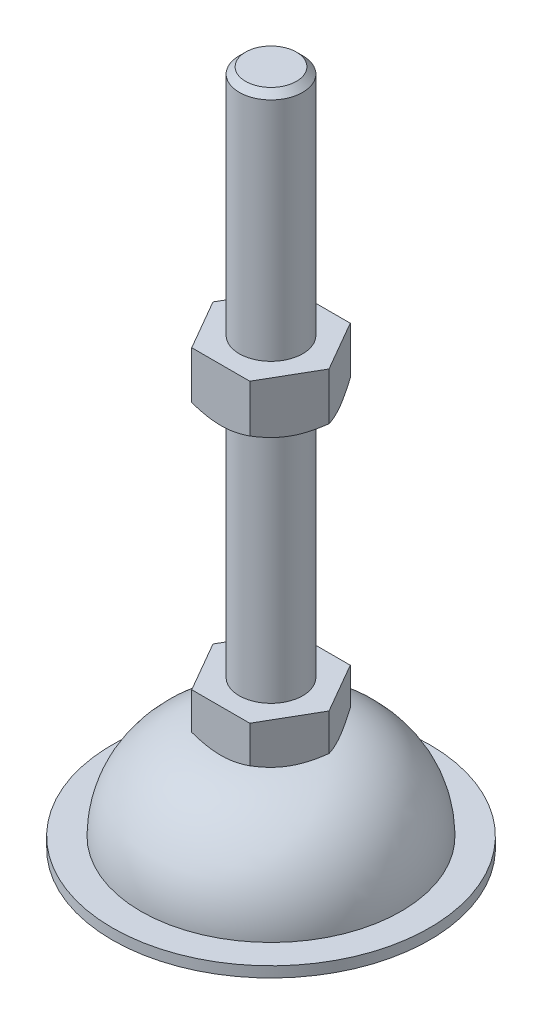
SolidWorks part; units mm, degrees
ref_plane "Front Plane" through (0, 0, 0) normal (0, 0, 1) x (1, 0, 0)
ref_plane "Top Plane" through (0, 0, 0) normal (0, 1, 0) x (1, 0, 0)
ref_plane "Right Plane" through (0, 0, 0) normal (1, 0, 0) x (0, 0, -1)
sketch "Sketch1" plane through (0, 0, 0) normal (1, 0, 0) x (0, 0, -1)
  line L0 (0, 0) -> (0, 128) construction
  line L1 (0, 128) -> (6, 128)
  line L2 (6, 128) -> (6, 20)
  line L3 (0, 0) -> (30, 0)
  line L4 (30, 0) -> (30, 2)
  line L5 (30, 2) -> (24.6, 2)
  line L6 (6, 20) -> (6.6, 20)
  line L8 (0, 84) -> (9.5, 84)
  line L9 (0, 84) -> (0, 74)
  line L10 (0, 74) -> (9.5, 74)
  line L11 (9.5, 84) -> (9.5, 74)
  line L12 (0, 28) -> (9.5, 28)
  line L13 (0, 28) -> (0, 20)
  line L14 (0, 20) -> (9.5, 20)
  line L15 (9.5, 28) -> (9.5, 20)
  arc A1 (24.6, 2) -> (6.6, 20) centre (6.6, 2) ccw
  point P18 (6, 74)
  dimension "D1" = 0.6
  dimension "M" = 12
  dimension "D" = 60
  dimension "e1" = 8
  dimension "e2" = 10
  dimension "E" = 18
  dimension "t" = 2
  dimension "B" = 19
  dimension "A" = 100
sketch "Sketch2" plane through (0, 0, 0) normal (1, 0, 0) x (0, 0, -1)
  line L0 (0, 128) -> (6, 128) construction
  line L1 (6, 128) -> (6, 20) construction
  line L2 (6, 20) -> (6.6, 20) construction
  line L3 (30, 2) -> (24.6, 2) construction
  line L4 (30, 0) -> (30, 2) construction
  line L5 (0, 0) -> (30, 0) construction
  line L6 (0, 128) -> (6, 128)
  line L7 (6, 128) -> (6, 20)
  line L8 (6, 20) -> (6.6, 20)
  line L9 (30, 2) -> (24.6, 2)
  line L10 (30, 0) -> (30, 2)
  line L11 (0, 0) -> (30, 0)
  line L12 (0, 128) -> (0, 0)
  arc A0 (24.6, 2) -> (6.6, 20) centre (6.6, 2) ccw construction
  arc A1 (24.6, 2) -> (6.6, 20) centre (6.6, 2) ccw
revolve "Revolve1" add sketch "Sketch2" angle 360 mid plane about L12
cosmetic thread "Cosmetic Thread1" parameters "D2"=11.9
chamfer "Chamfer1" distance 1.2 angle 45 1 edges at (0, 128, 6)
sketch "Sketch3" plane through (0, 0, 0) normal (0, 1, 0) x (1, 0, 0)
  line L1 (-10.9697, 0) -> (-5.4848, -9.5)
  line L2 (-5.4848, -9.5) -> (5.4848, -9.5)
  line L3 (5.4848, -9.5) -> (10.9697, 0)
  line L4 (10.9697, 0) -> (5.4848, 9.5)
  line L5 (5.4848, 9.5) -> (-5.4848, 9.5)
  line L6 (-5.4848, 9.5) -> (-10.9697, 0)
  circle A0 centre (0, 0) radius 9.5 construction
extrude "Boss-Extrude1" add sketch "Sketch3" along normal up to vertex (28 mm away) from vertex at 20 starting at point (0, 20, -9.5)
sketch "Sketch4" plane through (0, 0, 0) normal (0, 1, 0) x (1, 0, 0)
  line L1 (-5.4848, 9.5) -> (-10.9697, 0)
  line L2 (-10.9697, 0) -> (-5.4848, -9.5)
  line L3 (-5.4848, -9.5) -> (5.4848, -9.5)
  line L4 (5.4848, -9.5) -> (10.9697, 0)
  line L5 (10.9697, 0) -> (5.4848, 9.5)
  line L6 (5.4848, 9.5) -> (-5.4848, 9.5)
  circle A0 centre (0, 0) radius 9.5 construction
extrude "Boss-Extrude2" add sketch "Sketch4" along normal up to vertex (84 mm away) from vertex at 74 separate body starting at point (0, 74, -9.5)
sketch "Sketch5" plane through (0, 20, 0) normal (0, -1, 0) x (1, 0, 0)
  line L0 (6.2197, -10.7728) -> (4.75, -8.2272) construction
  circle A0 centre (0, 0) radius 12.4393
  circle A1 centre (0, 0) radius 9.5
  point P6 (5.4848, -9.5)
extrude "Cut-Extrude1" cut sketch "Sketch5" against normal blind 6.4 draft 55
sketch "Sketch6" plane through (0, 74, 0) normal (0, -1, 0) x (1, 0, 0)
  line L0 (6.2197, -10.7728) -> (4.75, -8.2272) construction
  circle A0 centre (0, 0) radius 9.5
  circle A1 centre (0, 0) radius 12.4393
  point P6 (5.4848, -9.5)
extrude "Cut-Extrude4" cut sketch "Sketch6" against normal blind 5 draft 55
